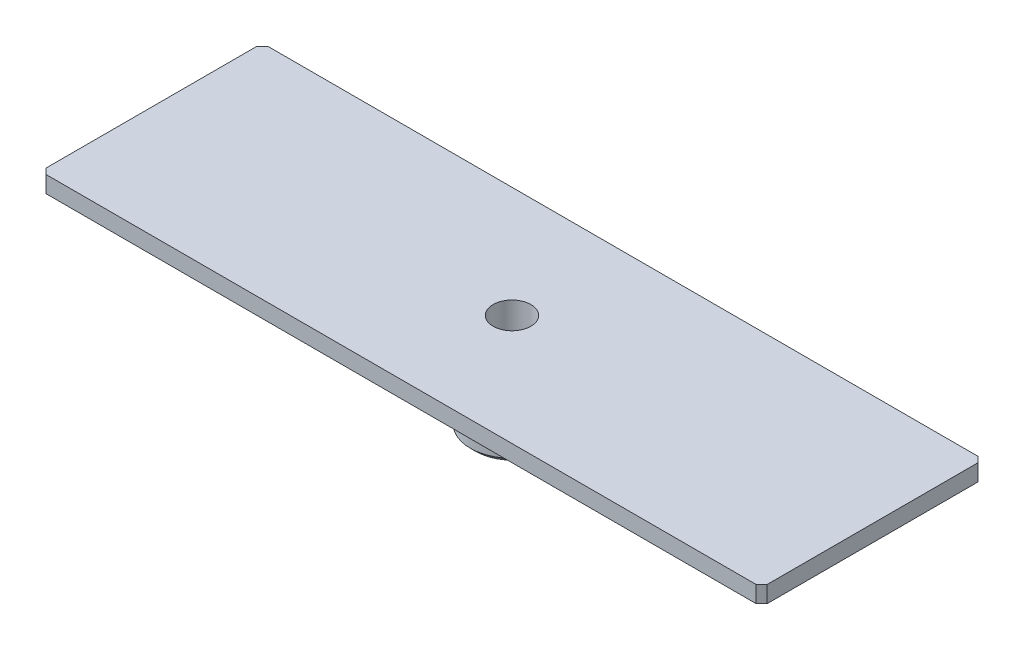
SolidWorks part; units mm, degrees
ref_plane "Front Plane" through (0, 0, 0) normal (0, 0, 1) x (1, 0, 0)
ref_plane "Top Plane" through (0, 0, 0) normal (0, 1, 0) x (1, 0, 0)
ref_plane "Right Plane" through (0, 0, 0) normal (1, 0, 0) x (0, 0, -1)
sketch "Sketch1" plane through (0, 0, 0) normal (0, 1, 0) x (1, 0, 0)
  circle A0 centre (0, 0) radius 7.5
  dimension "D1" = 15
extrude "Boss-Extrude1" add sketch "Sketch1" along normal blind 15
sketch "Sketch2" plane through (0, 15, 0) normal (0, 1, 0) x (1, 0, 0)
  line L1 (-65, 20) -> (65, 20)
  line L2 (-65, 20) -> (-65, -20)
  line L3 (-65, -20) -> (65, -20)
  line L4 (65, 20) -> (65, -20)
  line L5 (-65, 20) -> (65, -20) construction
  line L6 (-65, -20) -> (65, 20) construction
  point P0 (0, 0)
  dimension "D1" = 130
  dimension "D2" = 40
extrude "Boss-Extrude2" add sketch "Sketch2" along normal blind 3
hole_wizard "M8 Tapped Hole1" positions "Sketch3" profile "Sketch4" tap size "M8" standard "GB"
sketch "Sketch3" plane through (0, 0, 0) normal (0, -1, 0) x (-1, 0, 0)
  point P0 (0, 0)
sketch "Sketch4" plane through (0, 0, 0) normal (1, 0, 0) x (0, 0, -1)
  line L0 (0, 0) -> (0, 21.7929)
  line L1 (0, 21.7929) -> (3.4, 19.75)
  line L2 (3.4, 19.75) -> (3.4, 0)
  line L5 (3.4, 0) -> (0, 0)
  line L10 (0, 21.7929) -> (-3.4, 19.75) construction
  line L11 (0, -6.35) -> (0, 107.95) construction
  dimension "螺纹孔钻头直径" = 6.8
  dimension "螺纹孔钻头深度" = 19.75
  dimension "导头角度" = 118
cosmetic thread "Cosmetic Thread1" parameters "D1"=16, "D2"=8
chamfer "Chamfer1" distance 1 angle 45 6 edges at (0, 15, 7.5) (0, 0, 7.5) (65, 16.5, -20) (65, 16.5, 20) (-65, 16.5, 20) (-65, 16.5, -20)
